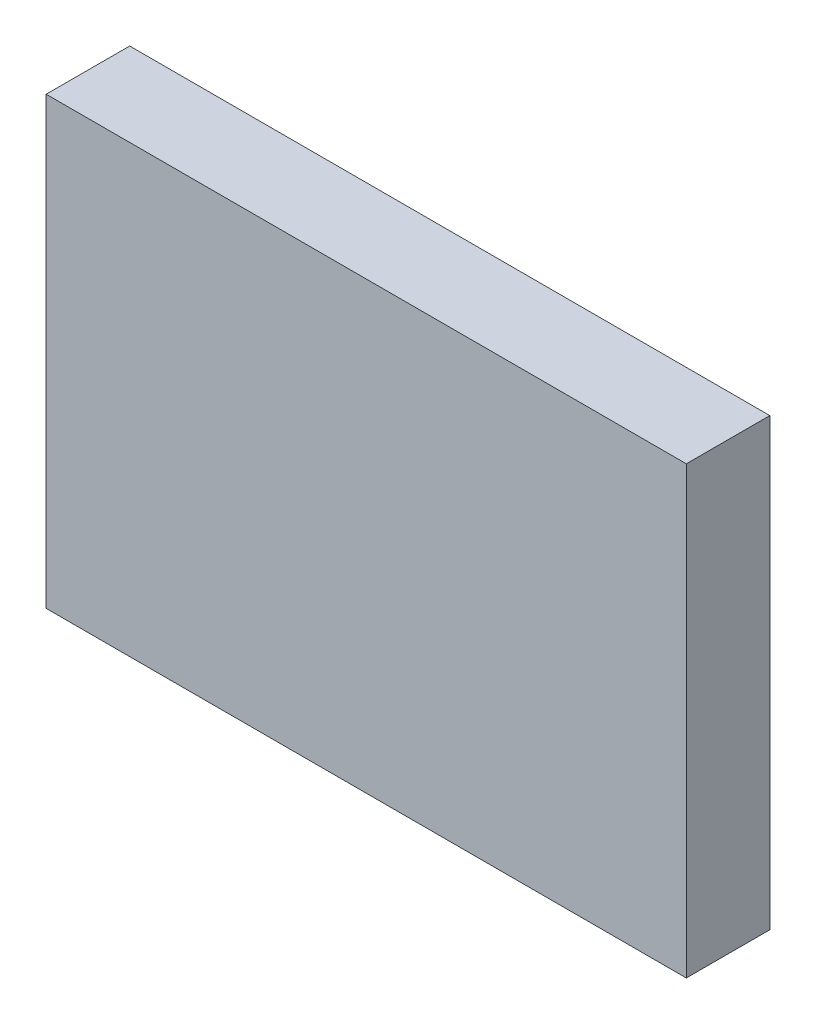
SolidWorks part; units mm, degrees
material "Q235B"
ref_plane "Front Plane" through (0, 0, 0) normal (0, 0, 1) x (1, 0, 0)
ref_plane "Top Plane" through (0, 0, 0) normal (0, 1, 0) x (1, 0, 0)
ref_plane "Right Plane" through (0, 0, 0) normal (1, 0, 0) x (0, 0, -1)
sketch "Sketch1" plane through (0, 0, 0) normal (0, 0, 1) x (1, 0, 0)
  line L1 (0, 0) -> (230, 0)
  line L2 (0, 0) -> (0, 160)
  line L3 (0, 160) -> (230, 160)
  line L4 (230, 0) -> (230, 160)
  dimension "D1" = 230
  dimension "D2" = 160
extrude "Boss-Extrude1" add sketch "Sketch1" along normal blind 30
